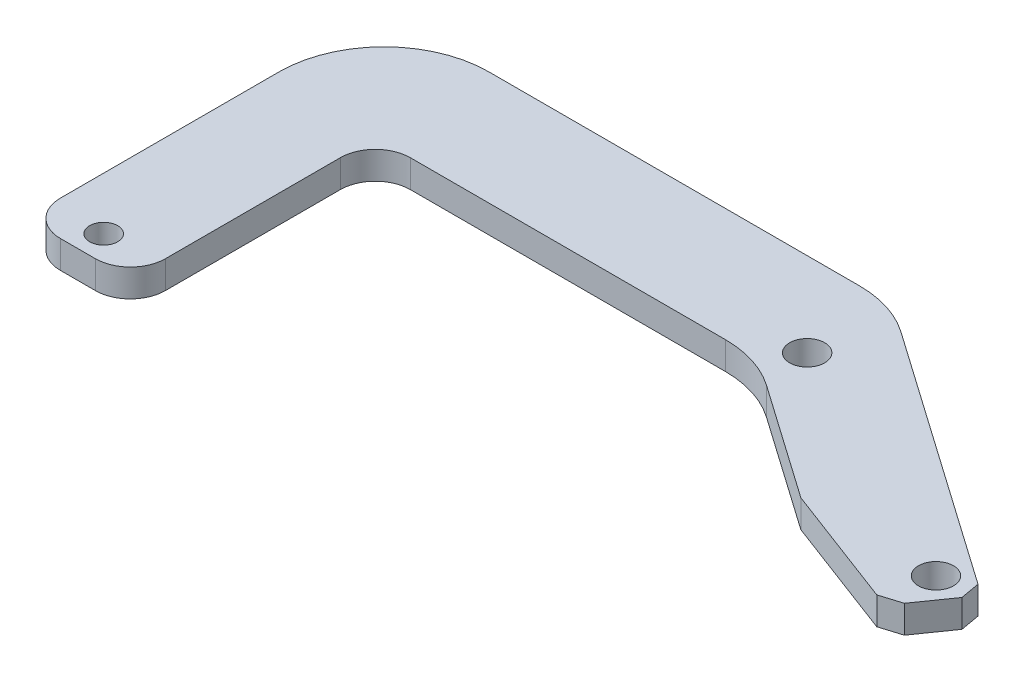
SolidWorks part; units mm, degrees
ref_plane "Plan de face" through (0, 0, 0) normal (0, 0, 1) x (1, 0, 0)
ref_plane "Plan de dessus" through (0, 0, 0) normal (0, 1, 0) x (1, 0, 0)
ref_plane "Plan de droite" through (0, 0, 0) normal (1, 0, 0) x (0, 0, -1)
sketch "Sketch1" plane through (0, 0, 0) normal (0, 1, 0) x (1, 0, 0)
  line L0 (149.6988, -34.8535) -> (116.9327, -11.9105)
  line L1 (99.7254, -6.485) -> (9.7254, -6.485)
  line L2 (-0.2746, -16.485) -> (-0.2746, -76.485)
  line L3 (196.3955, -30.9277) -> (122.8672, 20.5574)
  line L4 (105.6599, 25.9828) -> (-0.2746, 25.9828)
  line L5 (-0.2746, -76.485) -> (-30.2746, -76.485)
  line L6 (197.3778, -36.4986) -> (190.6063, -46.1694)
  line L7 (-30.2746, -76.485) -> (-30.2746, -4.0172)
  line L8 (206.6397, -47.6868) -> (138.1474, 0.2721) construction
  line L9 (184.5703, -48.0319) -> (149.6988, -34.8535)
  line L10 (-15.2746, -36.485) -> (-15.2746, -110.9721) construction
  line L11 (197.3778, -36.4986) -> (196.3955, -30.9277)
  line L12 (190.6063, -46.1694) -> (184.5703, -48.0319)
  arc A0 (-30.2746, -4.0172) -> (-0.2746, 25.9828) centre (-0.2746, -4.0172) cw
  arc A1 (116.9327, -11.9105) -> (99.7254, -6.485) centre (99.7254, -36.485) ccw
  arc A2 (122.8672, 20.5574) -> (105.6599, 25.9828) centre (105.6599, -4.0172) ccw
  arc A3 (-0.2746, -16.485) -> (9.7254, -6.485) centre (9.7254, -16.485) cw
  circle A4 centre (188.312, -34.8535) radius 5
  circle A5 centre (-15.2746, -69.1192) radius 4
  point P2 (199.6721, -33.222)
  point P16 (-0.2746, -6.485)
  point P21 (188.312, -49.446)
  dimension "D1" = 70
  dimension "D6" = 30
  dimension "D7" = 10
  dimension "D8" = 10
  dimension "D2" = 8
  dimension "D3" = 100
  dimension "D4" = 30
extrude "Boss.-Extru.1" add sketch "Sketch1" along normal blind 7.9
sketch "Sketch2" plane through (0, 0, 0) normal (0, -1, 0) x (1, 0, 0)
  line L0 (197.3778, 36.4986) -> (196.3955, 30.9277) construction
  circle A1 centre (114.7154, -1.9318) radius 5
  line B0 (196.3955, 30.9277) -> (122.8672, -20.5574) construction
  line B1 (122.8672, -20.5574) -> (114.7154, -1.9318) construction
  line B2 (197.3778, 36.4986) -> (196.3955, 30.9277) construction
  circle B3 centre (114.7154, -1.9318) radius 4 construction
  dimension "D1" = 10
sketch_block_instance "Bloc1-1"
sketch_block "Bloc1"
extrude "Cut-Extrude1" cut sketch "Sketch2" against normal through all contours A1
fillet "Fillet1" radius 10 2 edges at (-0.2746, 3.95, 76.485) (-30.2746, 3.95, 76.485)
